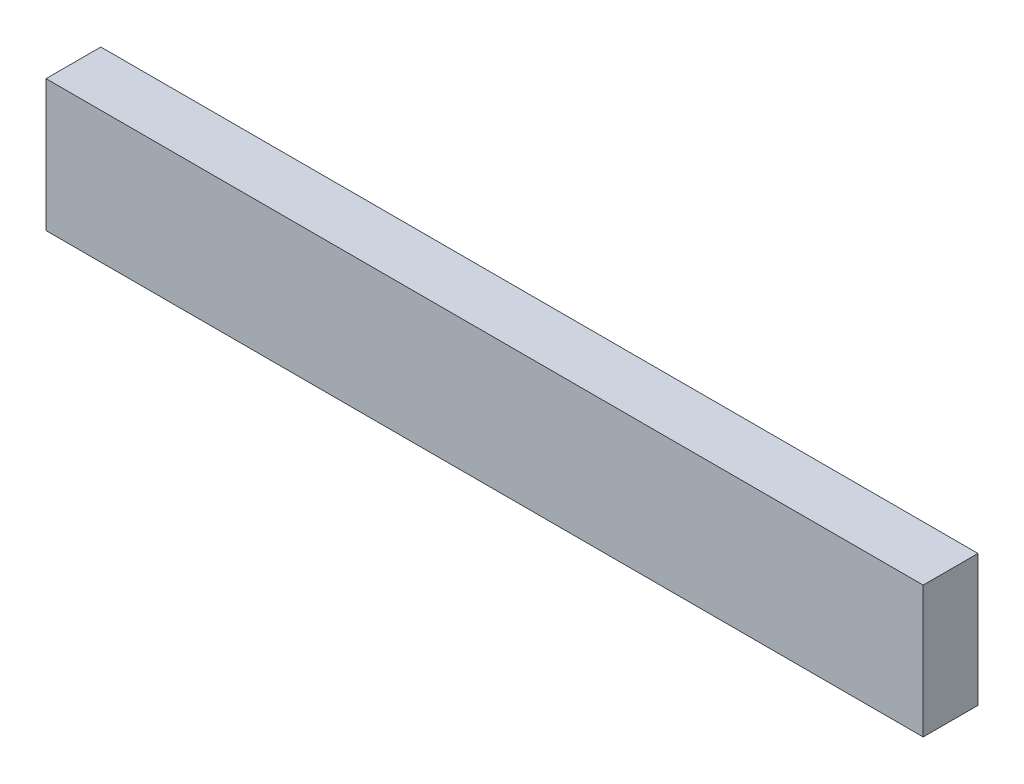
from build123d import *

# Parameters (mm, degrees)
SKETCH_1_W      = 800
SKETCH_1_H      = 120
EXTRUDE_1_DEPTH = 50


with BuildPart() as part:
    # 草图1 → 凸台-拉伸1 (new body)
    with BuildSketch(Plane.XY):
        with Locations((359.323818564, 53.766102462)):
            Rectangle(SKETCH_1_W, SKETCH_1_H)
    extrude(amount=EXTRUDE_1_DEPTH)


solid = part.part
